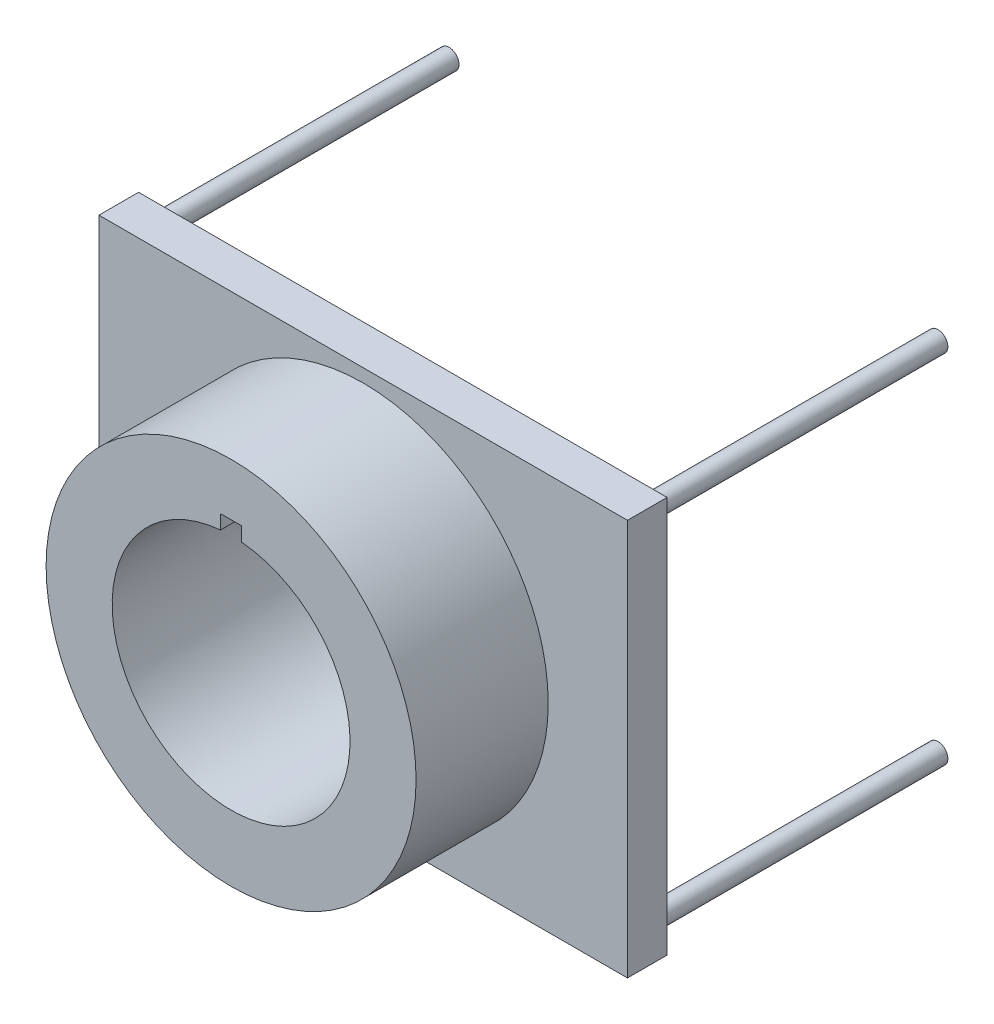
from build123d import *

# Parameters (mm, degrees)
SKETCH2_R           = 70
SKETCH2_R_2         = 45
BOSS_EXTRUDE1_DEPTH = 50
SKETCH3_W           = 200
SKETCH3_H           = 150
BOSS_EXTRUDE2_DEPTH = 15
SKETCH4_R           = 3.75
BOSS_EXTRUDE3_DEPTH = 110
SKETCH5_W           = 8
SKETCH5_H           = 7
CUT_EXTRUDE1_DEPTH  = 50
CUT_EXTRUDE3_START  = -70
SKETCH6_R           = 70
CUT_EXTRUDE3_DEPTH  = 70
SKETCH9_R           = 70
BOSS_EXTRUDE4_DEPTH = 15


with BuildPart() as part:
    # Sketch2 → Boss-Extrude1 (new body)
    with BuildSketch(Plane.XY):
        Circle(SKETCH2_R)
        Circle(SKETCH2_R_2, mode=Mode.SUBTRACT)
    extrude(amount=BOSS_EXTRUDE1_DEPTH)

    # Sketch3 → Boss-Extrude2 (add)
    with BuildSketch(Plane(origin=(0, 0, 0), x_dir=(-1, 0, 0), z_dir=(0, 0, -1))):
        Rectangle(SKETCH3_W, SKETCH3_H)
    extrude(amount=BOSS_EXTRUDE2_DEPTH)

    # Sketch4 → Boss-Extrude3 (add)
    with BuildSketch(Plane(origin=(0, 0, -15), x_dir=(-1, 0, 0), z_dir=(0, 0, -1))):
        with Locations(Location((-92.5, 67.5, 0), (0, 0, 180))):
            Circle(SKETCH4_R)
        with Locations(Location((92.5, 67.5, 0), (0, 0, 180))):
            Circle(SKETCH4_R)
        with Locations(Location((92.5, -67.5, 0), (0, 0, 180))):
            Circle(SKETCH4_R)
        with Locations(Location((-92.5, -67.5, 0), (0, 0, 180))):
            Circle(SKETCH4_R)
    extrude(amount=BOSS_EXTRUDE3_DEPTH)

    # Sketch5 → Cut-Extrude1 (cut)
    with BuildSketch(Plane.XY.offset(50)):
        with Locations((0, 46.68)):
            Rectangle(SKETCH5_W, SKETCH5_H)
    extrude(amount=-CUT_EXTRUDE1_DEPTH, mode=Mode.SUBTRACT)

    # Sketch6 → Cut-Extrude3 (cut)
    with BuildSketch(Plane.XY.offset(CUT_EXTRUDE3_START)):
        Circle(SKETCH6_R)
    extrude(amount=CUT_EXTRUDE3_DEPTH, mode=Mode.SUBTRACT)


with BuildPart() as cut_extrude3_piece_1:
    # of the separate pieces the step leaves, piece 1, a body of its own (cut_extrude3_pieces)
    add(part.part.solids().sort_by_distance((70, 0, 50))[0])

    # Sketch9 → Boss-Extrude4 (add)
    with BuildSketch(Plane(origin=(0, 0, 0), x_dir=(-1, 0, 0), z_dir=(0, 0, -1))):
        with Locations(Location((0, 0, 0), (0, 0, 180))):
            Circle(SKETCH9_R)
        with BuildLine():
            Line((4, 44.821869662), (4, 50.18))
            Line((4, 50.18), (-4, 50.18))
            Line((-4, 50.18), (-4, 44.821869662))
            ThreePointArc((-4, 44.821869662), (0, -45), (4, 44.821869662))
        make_face(mode=Mode.SUBTRACT)
    extrude(amount=BOSS_EXTRUDE4_DEPTH)


with BuildPart() as cut_extrude3_piece_2:
    # of the separate pieces the step leaves, piece 2, a body of its own (cut_extrude3_pieces)
    add(part.part.solids().sort_by_distance((100, -75, 0))[0])


solid = Compound([cut_extrude3_piece_1.part, cut_extrude3_piece_2.part])
